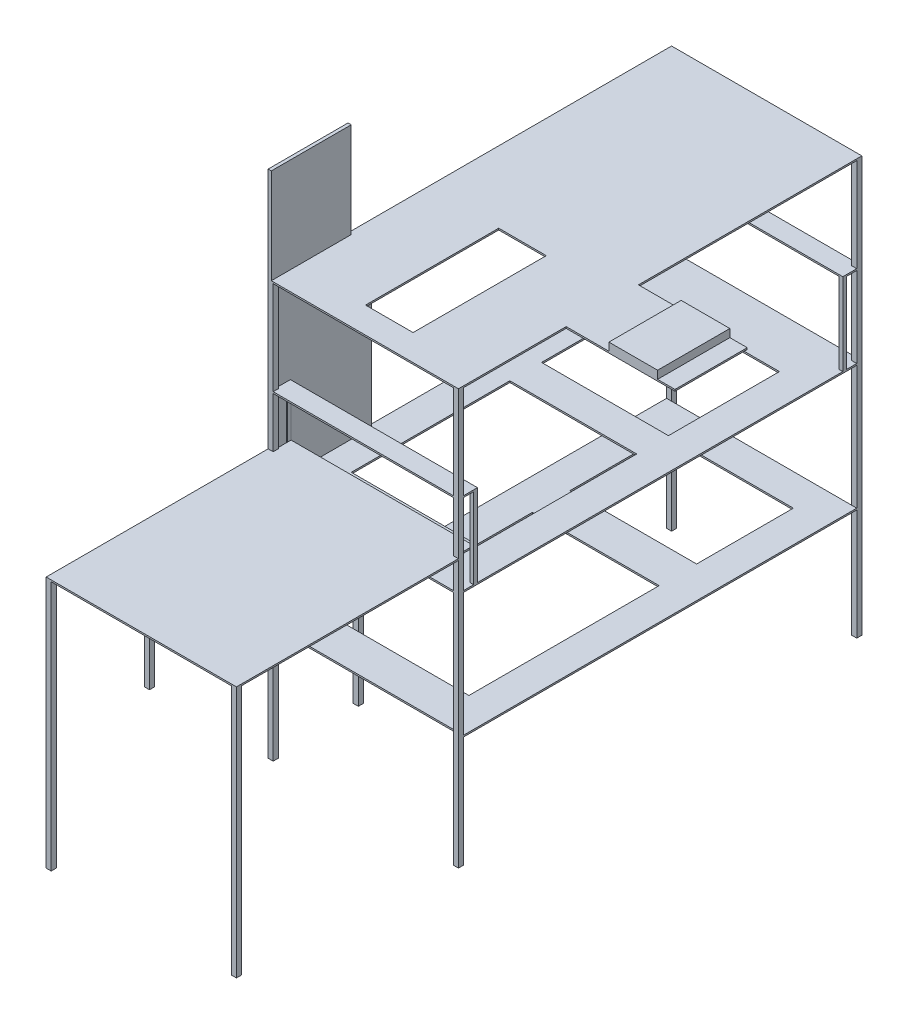
from build123d import *

# Parameters (mm, degrees)
SKETCH_4_W               = 16
SKETCH_4_H               = 16
EXTRUDE_1_DEPTH          = 1309
EXTRUDE_1_2_DEPTH        = 1309
EXTRUDE_1_3_DEPTH        = 1309
EXTRUDE_1_4_DEPTH        = 1309
SKETCH_5_W               = 599.732743224
SKETCH_5_H               = 1240
EXTRUDE_2_DEPTH          = 5
SKETCH_7_W               = 16
SKETCH_7_H               = 16
EXTRUDE_3_DEPTH          = 400
SKETCH_8_W               = 406
SKETCH_8_H               = 300
EXTRUDE_4_DEPTH          = 5
SKETCH_9_W               = 600
SKETCH_9_H               = 1272
EXTRUDE_5_DEPTH          = 5
SKETCH_10_W              = 600
SKETCH_10_H              = 60
EXTRUDE_6_DEPTH          = 5
EXTRUDE_7_REACH          = 1769.631
SKETCH_11_W              = 12
SKETCH_11_H              = 12
MIRROR_3_COPY_1_REACH    = 1769.631
MIRROR_3_COPY_1_SKETCH_W = 12
MIRROR_3_COPY_1_SKETCH_H = 12
SKETCH_12_W              = 600
SKETCH_12_H              = 1272
EXTRUDE_8_DEPTH          = 5
EXTRUDE_START            = 90
SKETCH_18_W              = 575.732743224
SKETCH_18_H              = 60
EXTRUDE_11_DEPTH         = 5
SKETCH_19_W              = 600
SKETCH_19_H              = 5
EXTRUDE_12_DEPTH         = 700
SKETCH_21_W              = 400
SKETCH_21_H              = 350
CUT_EXTRUDE_4_DEPTH      = 10
SKETCH_22_W              = 16
SKETCH_22_H              = 16
EXTRUDE_14_DEPTH         = 790
SKETCH_23_W              = 400
SKETCH_23_H              = 600
CUT_EXTRUDE_5_DEPTH      = 1864.366845256
SKETCH_24_W              = 150
SKETCH_24_H              = 420
CUT_EXTRUDE_6_DEPTH      = 10
SKETCH_25_W              = 400
SKETCH_25_H              = 305
CUT_EXTRUDE_7_DEPTH      = 10
EXTRUDE_15_REACH         = 1845.208
SKETCH_26_W              = 16
SKETCH_26_H              = 16
PATTERN_LINEAR_1_COUNT   = 2
PATTERN_LINEAR_1_PITCH   = 600
SKETCH_27_W              = 400
SKETCH_27_H              = 5
CUT_EXTRUDE_8_DEPTH      = 150
SKETCH_28_W              = 300
SKETCH_28_H              = 554
EXTRUDE_16_DEPTH         = 10
SKETCH_29_W              = 316
SKETCH_29_H              = 300
EXTRUDE_17_DEPTH         = 10
SKETCH_30_W              = 64
SKETCH_30_H              = 300
CUT_EXTRUDE_9_DEPTH      = 10
SKETCH_35_W              = 343.096096547
SKETCH_35_H              = 227.820151314
EXTRUDE_18_DEPTH         = 5
SKETCH_36_W              = 153.4970354
SKETCH_36_H              = 227.820151314
EXTRUDE_19_DEPTH         = 25


with BuildPart() as part:
    # 草图4 → 凸台-拉伸1 (new body)
    with BuildSketch(Plane(origin=(0, 0, 0), x_dir=(1, 0, 0), z_dir=(0, 1, 0))):
        Rectangle(SKETCH_4_W, SKETCH_4_H)
    extrude(amount=EXTRUDE_1_DEPTH)



with BuildPart() as body_2:
    # 草图4 → Extrude 1 2 (new body)
    with BuildSketch(Plane(origin=(0, 0, 0), x_dir=(1, 0, 0), z_dir=(0, 1, 0))):
        with Locations((0, 1256)):
            Rectangle(SKETCH_4_W, SKETCH_4_H)
    extrude(amount=EXTRUDE_1_2_DEPTH)


with BuildPart() as body_3:
    # 草图4 → Extrude 1 3 (new body)
    with BuildSketch(Plane(origin=(0, 0, 0), x_dir=(1, 0, 0), z_dir=(0, 1, 0))):
        with Locations((-584, 0)):
            Rectangle(SKETCH_4_W, SKETCH_4_H)
    extrude(amount=EXTRUDE_1_3_DEPTH)


with BuildPart() as body_4:
    # 草图4 → Extrude 1 4 (new body)
    with BuildSketch(Plane(origin=(0, 0, 0), x_dir=(1, 0, 0), z_dir=(0, 1, 0))):
        with Locations((-584, 1256)):
            Rectangle(SKETCH_4_W, SKETCH_4_H)
    extrude(amount=EXTRUDE_1_4_DEPTH)


with BuildPart() as part_1:
    add(part.part)

    add(body_2.part)  # 凸台-拉伸2 merges body 2

    add(body_3.part)  # 凸台-拉伸2 merges body 3

    add(body_4.part)  # 凸台-拉伸2 merges body 4
    # 草图5 → 凸台-拉伸2 (add)
    with BuildSketch(Plane(origin=(0, 350, 0), x_dir=(1, 0, 0), z_dir=(0, 1, 0))):
        with Locations((-291.866371612, 628)):
            Rectangle(SKETCH_5_W, SKETCH_5_H)
    extrude(amount=EXTRUDE_2_DEPTH)



with BuildPart() as body_2_2:
    # 草图7 → 凸台-拉伸3 (new body)
    with BuildSketch(Plane(origin=(0, 0, 0), x_dir=(1, 0, 0), z_dir=(0, 1, 0))):
        with Locations((-974, 0)):
            Rectangle(SKETCH_7_W, SKETCH_7_H)
    extrude(amount=EXTRUDE_3_DEPTH)


with BuildPart() as part_2:
    add(part_1.part)

    add(body_2_2.part)  # 凸台-拉伸4 merges body 2 2
    # 草图8 → 凸台-拉伸4 (add)
    with BuildSketch(Plane(origin=(0, 400, 0), x_dir=(1, 0, 0), z_dir=(0, 1, 0))):
        with Locations((-779, 142)):
            Rectangle(SKETCH_8_W, SKETCH_8_H)
    extrude(amount=-EXTRUDE_4_DEPTH)

    # 草图9 → 凸台-拉伸5 (add)
    with BuildSketch(Plane(origin=(0, 750, 0), x_dir=(-1, 0, 0), z_dir=(0, -1, 0))):
        with Locations((292, 628)):
            Rectangle(SKETCH_9_W, SKETCH_9_H)
    extrude(amount=EXTRUDE_5_DEPTH)

    # 草图10 → 凸台-拉伸6 (add)
    with BuildSketch(Plane(origin=(0, 1009, 0), x_dir=(-1, 0, 0), z_dir=(0, -1, 0))):
        with Locations((292, 22)):
            Rectangle(SKETCH_10_W, SKETCH_10_H)
    extrude_6 = extrude(amount=EXTRUDE_6_DEPTH)

    # 镜向1: 凸台-拉伸6 across plane
    add(extrude_6.mirror(Plane.XY.offset(-628)))

    # 草图11 → 凸台-拉伸7 (add, up to next)
    with BuildSketch(Plane(origin=(0, 750, 0), x_dir=(1, 0, 0), z_dir=(0, 1, 0)), mode=Mode.PRIVATE) as extrude_7_sk1:
        with Locations((2, 46)):
            Rectangle(SKETCH_11_W, SKETCH_11_H)
    extrude_7_tool1 = extrude(extrude_7_sk1.sketch, amount=EXTRUDE_7_REACH, mode=Mode.PRIVATE) - part_2.part
    extrude_7 = extrude_7_tool1.solids().sort_by_distance((2, 750, -46))[0]
    add(extrude_7)

    # 镜向2: 凸台-拉伸7 across plane
    add(extrude_7.mirror(Plane(origin=(-291.866371612, 0, 0), x_dir=(0, 0, 1), z_dir=(1, 0, 0))))

    # 镜向3: 凸台-拉伸7 across plane
    add(extrude_7.mirror(Plane.XY.offset(-628)))

    # 镜向3 copy 1 sketch → 镜向3 copy 1 (add, up to next)
    with BuildSketch(Plane(origin=(-583.732743224, 750, -1256), x_dir=(-1, 0, 0), z_dir=(0, 1, 0)), mode=Mode.PRIVATE) as mirror_3_copy_1_sk1:
        with Locations((2, 46)):
            Rectangle(MIRROR_3_COPY_1_SKETCH_W, MIRROR_3_COPY_1_SKETCH_H)
    mirror_3_copy_1_tool1 = extrude(mirror_3_copy_1_sk1.sketch, amount=MIRROR_3_COPY_1_REACH, mode=Mode.PRIVATE) - part_2.part
    add(mirror_3_copy_1_tool1.solids().sort_by_distance((-585.732743224, 750, -1210))[0])

    # 草图12 → 凸台-拉伸8 (add)
    with BuildSketch(Plane(origin=(0, 1309, 0), x_dir=(1, 0, 0), z_dir=(0, 1, 0))):
        with Locations((-292, 628)):
            Rectangle(SKETCH_12_W, SKETCH_12_H)
    extrude(amount=-EXTRUDE_8_DEPTH)

    # 草图18 → 凸台-拉伸11 (add)
    with BuildSketch(Plane(origin=(0, 750, 0), x_dir=(1, 0, 0), z_dir=(0, 1, 0)).offset(EXTRUDE_START)):
        with Locations((-291.866371612, 22)):
            Rectangle(SKETCH_18_W, SKETCH_18_H)
    extrude(amount=EXTRUDE_11_DEPTH)

    # 草图19 → 凸台-拉伸12 (add)
    with BuildSketch(Plane.XY.offset(8)):
        with Locations((-292, 842.5)):
            Rectangle(SKETCH_19_W, SKETCH_19_H)
    extrude(amount=EXTRUDE_12_DEPTH)

    # 草图21 → 切除-拉伸4 (cut)
    with BuildSketch(Plane(origin=(0, 750, 0), x_dir=(1, 0, 0), z_dir=(0, 1, 0))):
        with Locations((-291.866371612, 929)):
            Rectangle(SKETCH_21_W, SKETCH_21_H)
    cut_extrude_4 = extrude(amount=-CUT_EXTRUDE_4_DEPTH, mode=Mode.SUBTRACT)

    # 草图22 → 凸台-拉伸14 (add)
    with BuildSketch(Plane.XZ.offset(-840)):
        with Locations((-584, 700)):
            Rectangle(SKETCH_22_W, SKETCH_22_H)
        with Locations((0, 700)):
            Rectangle(SKETCH_22_W, SKETCH_22_H)
    extrude(amount=EXTRUDE_14_DEPTH)

    # 草图23 → 切除-拉伸5 (cut, through all)
    with BuildSketch(Plane(origin=(0, 355, 0), x_dir=(1, 0, 0), z_dir=(0, 1, 0))):
        with Locations((-292, 425)):
            Rectangle(SKETCH_23_W, SKETCH_23_H)
    extrude(amount=-CUT_EXTRUDE_5_DEPTH, mode=Mode.SUBTRACT)

    # 草图24 → 切除-拉伸6 (cut)
    with BuildSketch(Plane(origin=(0, 1309, 0), x_dir=(1, 0, 0), z_dir=(0, 1, 0))):
        with Locations((-292, 284)):
            Rectangle(SKETCH_24_W, SKETCH_24_H)
    extrude(amount=-CUT_EXTRUDE_6_DEPTH, mode=Mode.SUBTRACT)

    # 草图25 → 切除-拉伸7 (cut)
    with BuildSketch(Plane(origin=(0, 355, 0), x_dir=(1, 0, 0), z_dir=(0, 1, 0))):
        with Locations((-292, 995.5)):
            Rectangle(SKETCH_25_W, SKETCH_25_H)
    extrude(amount=-CUT_EXTRUDE_7_DEPTH, mode=Mode.SUBTRACT)

    # 凸台-拉伸15: up to this face of the body (flat: up to its plane)
    extrude_15_end = Plane(part_2.part.faces().sort_by_distance((-974, 0, 0))[0])
    # 草图26 → 凸台-拉伸15 (add, up to the picked face)
    with BuildSketch(Plane.XZ.offset(-395), mode=Mode.PRIVATE) as extrude_15_sk1:
        with Locations((-974, -284)):
            Rectangle(SKETCH_26_W, SKETCH_26_H)
    extrude_15_tool1 = split(extrude(extrude_15_sk1.sketch, amount=EXTRUDE_15_REACH, mode=Mode.PRIVATE), bisect_by=extrude_15_end, keep=Keep.BOTH, mode=Mode.PRIVATE)
    # 草图26 → 凸台-拉伸15 (add, up to the picked face)
    with BuildSketch(Plane.XZ.offset(-395), mode=Mode.PRIVATE) as extrude_15_sk2:
        with Locations((-599.732743224, -284)):
            Rectangle(SKETCH_26_W, SKETCH_26_H)
    extrude_15_tool2 = split(extrude(extrude_15_sk2.sketch, amount=EXTRUDE_15_REACH, mode=Mode.PRIVATE), bisect_by=extrude_15_end, keep=Keep.BOTH, mode=Mode.PRIVATE)
    add(extrude_15_tool1.solids().sort_by(Axis((-974, 395, -284), (0, -1, 0)))[0])
    add(extrude_15_tool2.solids().sort_by(Axis((-599.732743, 395, -284), (0, -1, 0)))[0])

    # 阵列(线性)1: 切除-拉伸4 ×2
    with Locations(*[(0, 0, i * PATTERN_LINEAR_1_PITCH) for i in range(1, PATTERN_LINEAR_1_COUNT)]):
        add(cut_extrude_4, mode=Mode.SUBTRACT)

    # 草图27 → 切除-拉伸8 (cut)
    with BuildSketch(Plane.XY.offset(-504)):
        with Locations((-291.866371612, 747.5)):
            Rectangle(SKETCH_27_W, SKETCH_27_H)
    extrude(amount=-CUT_EXTRUDE_8_DEPTH, mode=Mode.SUBTRACT)

    # 草图28 → 凸台-拉伸16 (add)
    with BuildSketch(Plane.ZY.offset(592)):
        with Locations((-158, 1027)):
            Rectangle(SKETCH_28_W, SKETCH_28_H)
    extrude(amount=-EXTRUDE_16_DEPTH)

    # 草图29 → 凸台-拉伸17 (add)
    with BuildSketch(Plane.ZY.offset(592)):
        with Locations((-150, 1459)):
            Rectangle(SKETCH_29_W, SKETCH_29_H)
    extrude(amount=-EXTRUDE_17_DEPTH)

    # 草图30 → 切除-拉伸9 (cut)
    with BuildSketch(Plane.ZY.offset(592)):
        with Locations((-276, 1459)):
            Rectangle(SKETCH_30_W, SKETCH_30_H)
    extrude(amount=-CUT_EXTRUDE_9_DEPTH, mode=Mode.SUBTRACT)

    # 草图35 → 凸台-拉伸18 (add)
    with BuildSketch(Plane(origin=(0, 1309, 0), x_dir=(1, 0, 0), z_dir=(0, 1, 0))):
        with Locations((179.548048274, 445.599054932)):
            Rectangle(SKETCH_35_W, SKETCH_35_H)
    extrude(amount=-EXTRUDE_18_DEPTH)

    # 草图36 → 凸台-拉伸19 (add)
    with BuildSketch(Plane(origin=(0, 1309, 0), x_dir=(1, 0, 0), z_dir=(0, 1, 0))):
        with Locations((219.510855053, 445.599054932)):
            Rectangle(SKETCH_36_W, SKETCH_36_H)
    extrude(amount=EXTRUDE_19_DEPTH)


solid = part_2.part
